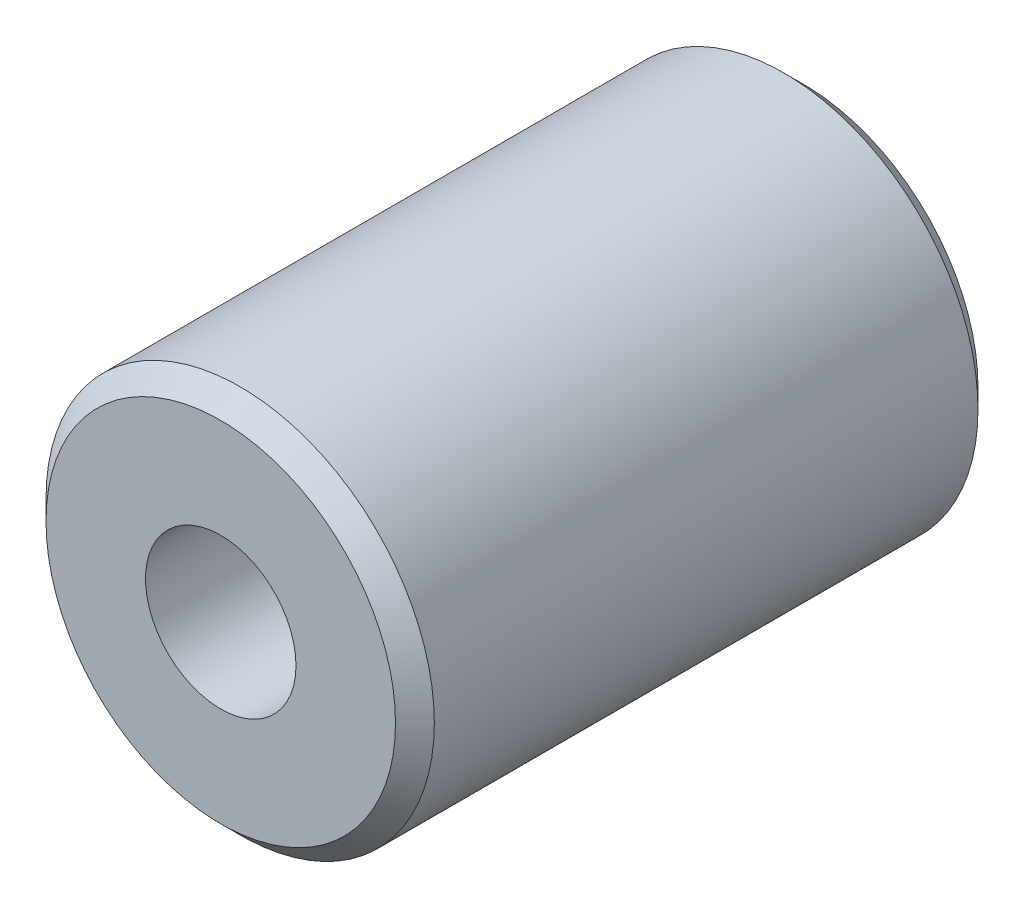
SolidWorks part; units mm, degrees
ref_plane "Front Plane" through (0, 0, 0) normal (0, 0, 1) x (1, 0, 0)
ref_plane "Top Plane" through (0, 0, 0) normal (0, 1, 0) x (1, 0, 0)
ref_plane "Right Plane" through (0, 0, 0) normal (1, 0, 0) x (0, 0, -1)
sketch "Sketch1" plane through (0, 0, 0) normal (0, 0, 1) x (1, 0, 0)
  circle A0 centre (0, 0) radius 20
  dimension "D1" = 40
extrude "Boss-Extrude1" add sketch "Sketch1" along normal mid plane 60
chamfer "Chamfer1" distance 2 angle 45 2 edges at (20, 0, -30) (20, 0, 30)
hole_wizard "M18 Tapped Hole1" positions "Sketch2" profile "Sketch3" tap size "M18" standard "GB" end condition through all
sketch "Sketch2" plane through (0, 0, 30) normal (0, 0, 1) x (1, 0, 0)
  point P0 (0, 0)
sketch "Sketch3" plane through (0, 0, 30) normal (1, 0, 0) x (0, -1, 0)
  line L0 (0, 0) -> (0, 60)
  line L1 (0, 60) -> (7.75, 60)
  line L2 (7.75, 60) -> (7.75, 0)
  line L5 (7.75, 0) -> (0, 0)
  line L11 (0, -6.35) -> (0, 107.95) construction
  dimension "通孔螺纹孔钻头直径" = 15.5
  dimension "通孔螺纹孔钻头深度" = 60
cosmetic thread "Cosmetic Thread1" parameters "D2"=18
